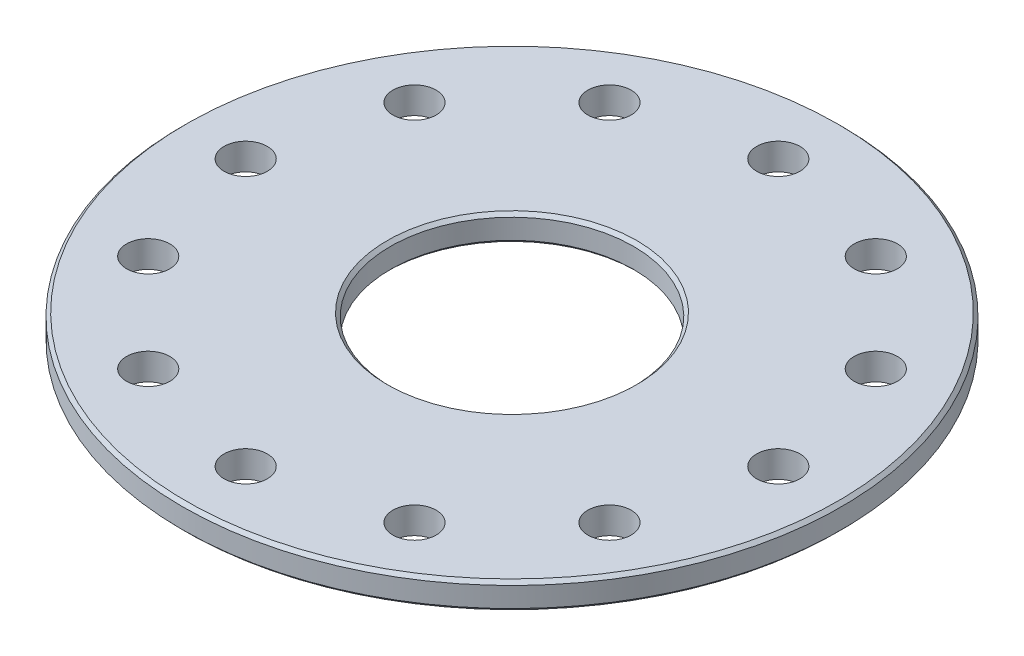
from build123d import *

# Parameters (mm, degrees)
SKETCH_1_R      = 99
SKETCH_1_R_2    = 6.5
SKETCH_1_R_3    = 36.5
EXTRUDE_1_DEPTH = 8
CHAMFER_1_SIZE  = 1


with BuildPart() as part:
    # 草图1 → 凸台-拉伸1 (new body)
    with BuildSketch(Plane(origin=(0, 87, 0), x_dir=(1, 0, 0), z_dir=(0, 1, 0))):
        with Locations(Location((0, 0, 0), (0, 0, 90))):
            Circle(SKETCH_1_R)
        with Locations(Location((-80, 0, 0), (0, 0, 90))):
            Circle(SKETCH_1_R_2, mode=Mode.SUBTRACT)
        with Locations(Location((40, 69.282032303, 0), (0, 0, 90))):
            Circle(SKETCH_1_R_2, mode=Mode.SUBTRACT)
        with Locations(Location((-69.282032733, 40, 0), (0, 0, 90))):
            Circle(SKETCH_1_R_2, mode=Mode.SUBTRACT)
        with Locations(Location((-69.282032733, -39.999999255, 0), (0, 0, 90))):
            Circle(SKETCH_1_R_2, mode=Mode.SUBTRACT)
        with Locations(Location((0, 80, 0), (0, 0, 90))):
            Circle(SKETCH_1_R_2, mode=Mode.SUBTRACT)
        with Locations(Location((69.282032302, -39.999999255, 0), (0, 0, 90))):
            Circle(SKETCH_1_R_2, mode=Mode.SUBTRACT)
        with Locations(Location((-40, 69.282032303, 0), (0, 0, 90))):
            Circle(SKETCH_1_R_2, mode=Mode.SUBTRACT)
        with Locations(Location((0, -80, 0), (0, 0, 90))):
            Circle(SKETCH_1_R_2, mode=Mode.SUBTRACT)
        with Locations(Location((40, -69.282032303, 0), (0, 0, 90))):
            Circle(SKETCH_1_R_2, mode=Mode.SUBTRACT)
        with Locations(Location((69.282032302, 40, 0), (0, 0, 90))):
            Circle(SKETCH_1_R_2, mode=Mode.SUBTRACT)
        with Locations(Location((-40, -69.282032303, 0), (0, 0, 90))):
            Circle(SKETCH_1_R_2, mode=Mode.SUBTRACT)
        with Locations(Location((80, 0, 0), (0, 0, 90))):
            Circle(SKETCH_1_R_2, mode=Mode.SUBTRACT)
        with Locations(Location((0, 0, 0), (0, 0, 90))):
            Circle(SKETCH_1_R_3, mode=Mode.SUBTRACT)
    extrude(amount=-EXTRUDE_1_DEPTH)

    # 倒角1
    chamfer_1_edges = [part.edges().sort_by_distance(p)[0] for p in [
        (0, 87, 99),
        (0, 79, 99),
        (0, 79, 36.5),
        (0, 87, 36.5),
    ]]
    chamfer(chamfer_1_edges, length=CHAMFER_1_SIZE)


solid = part.part
